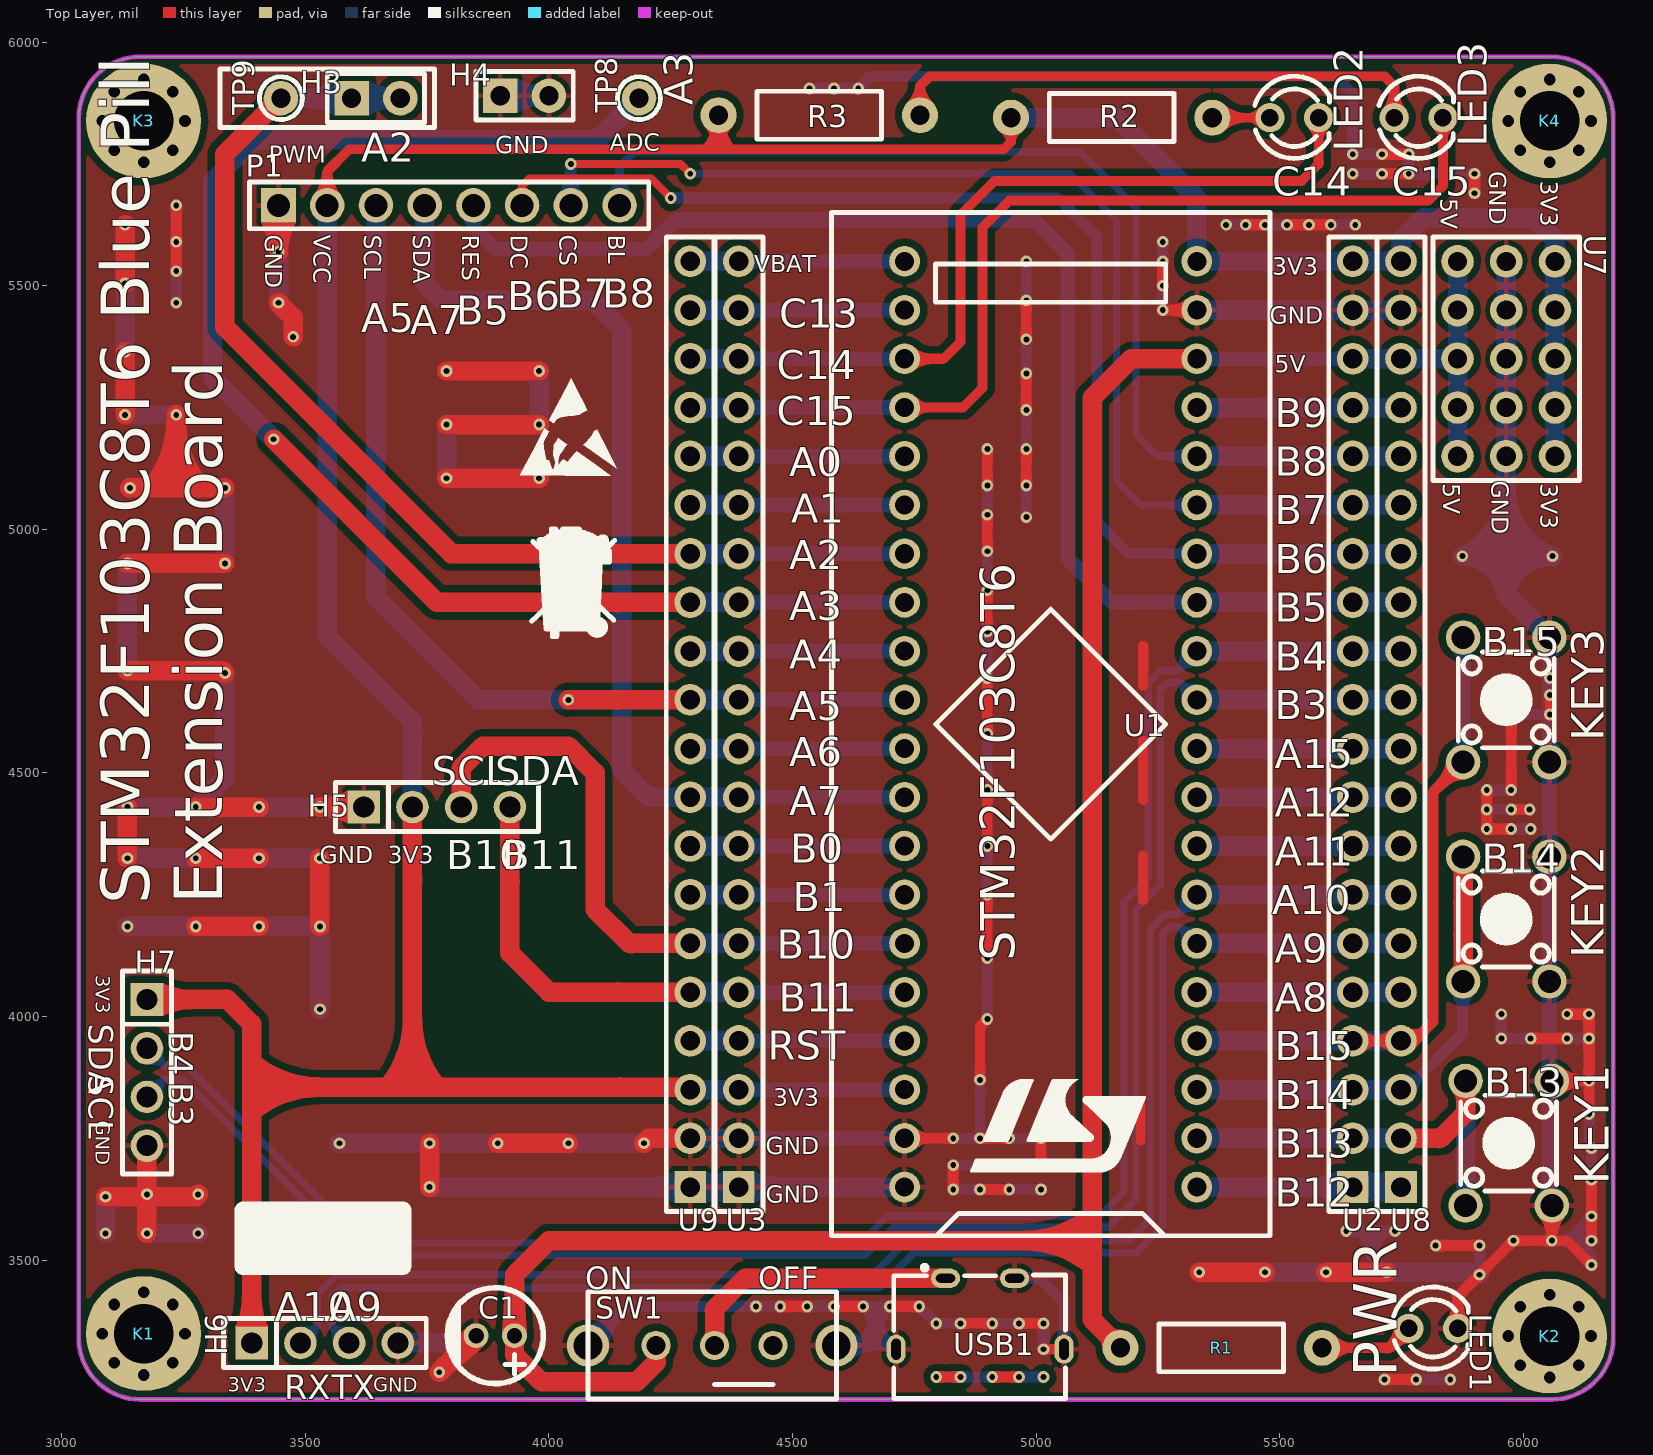
[diagram p0: Top Layer view]
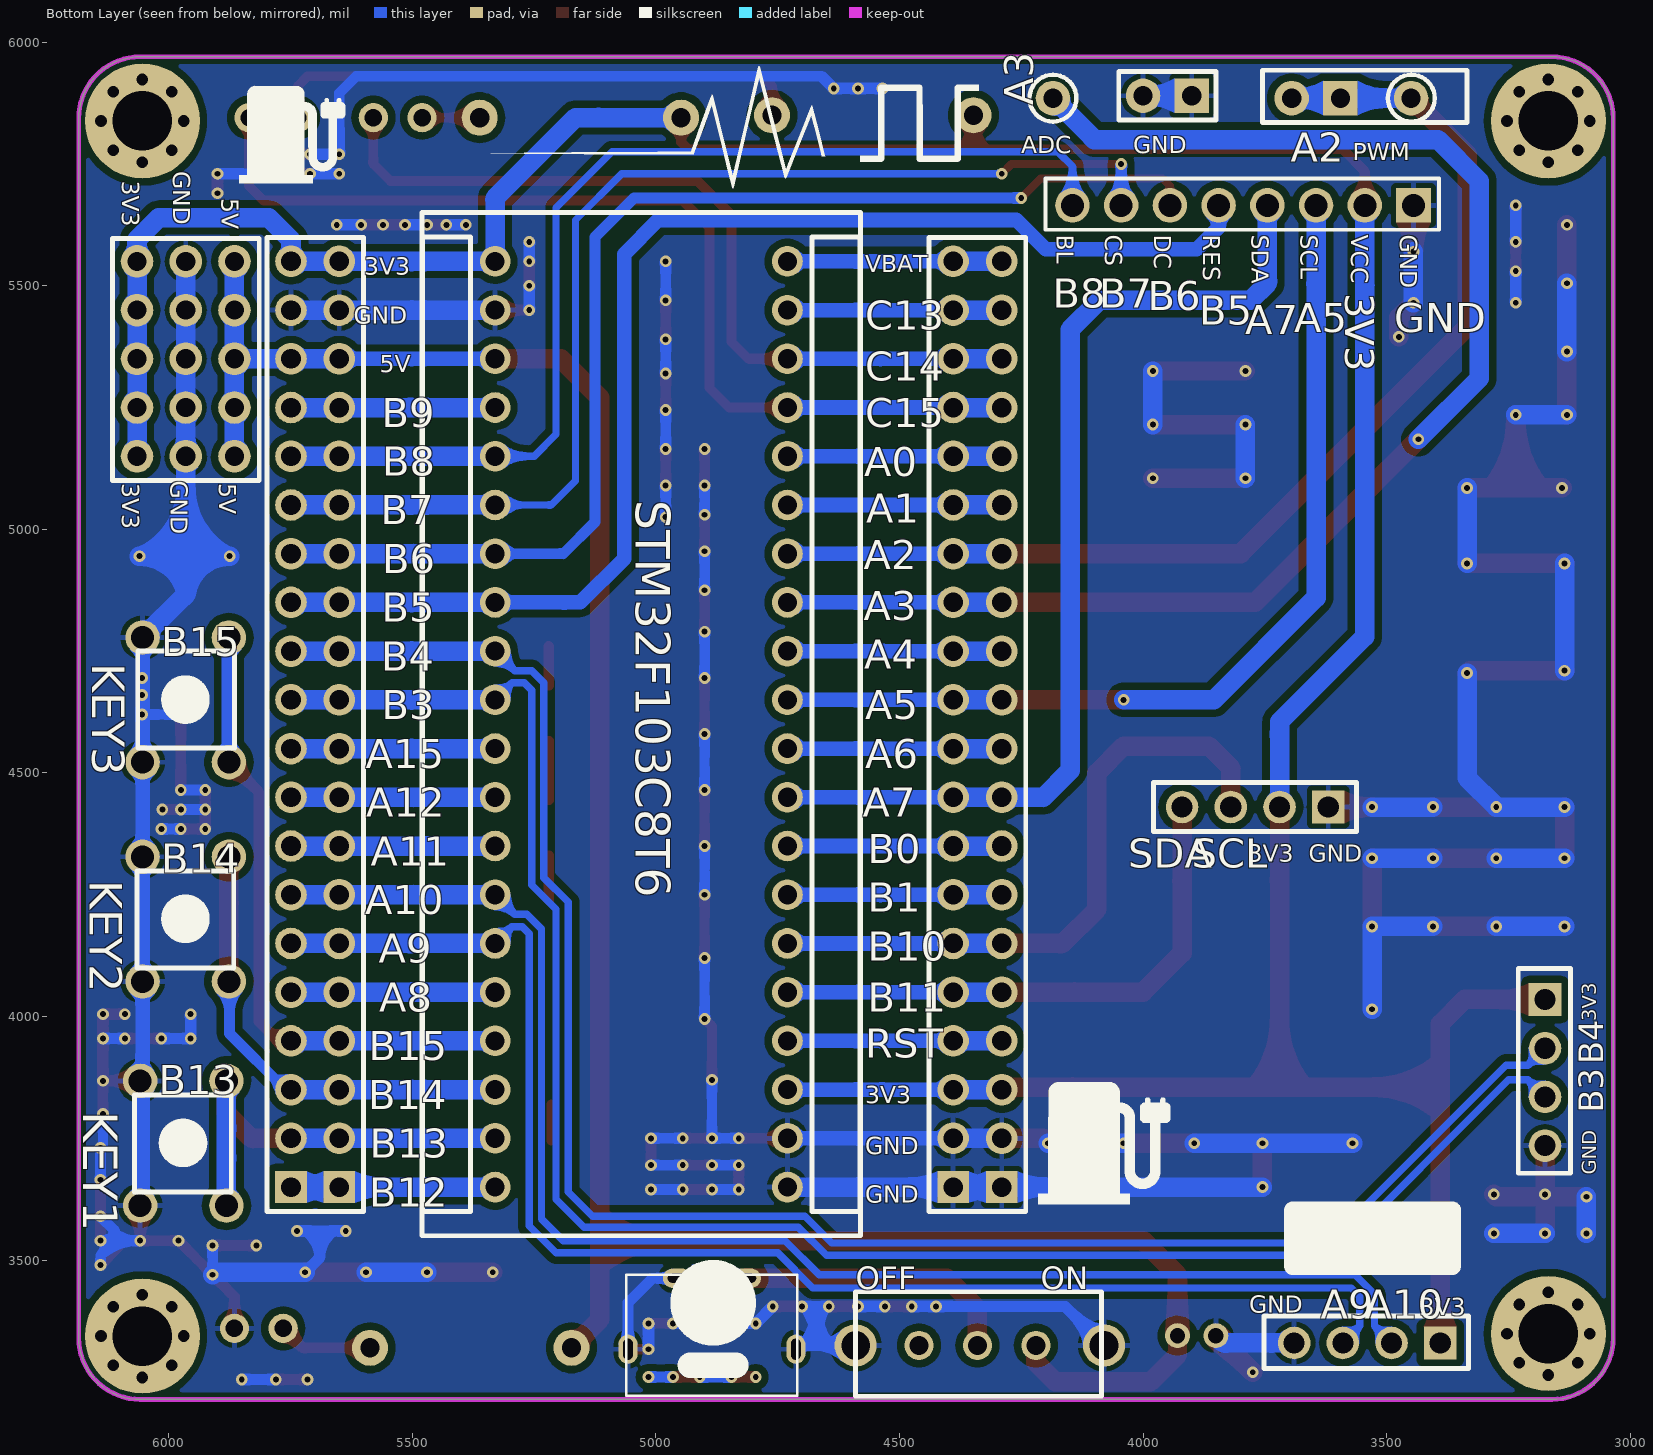
[diagram p1: Bottom Layer view, seen from below]
# Altium PCB MISC75409.pcbdoc
Units mil, origin at the board's own origin, x right, y up, seen from the top; angles counter-clockwise.
Board outline 3149.61 x 2755.91 mil, 2 copper layers (Top Layer, Bottom Layer), stack 62.206 mil thick; 30 components, 42 nets, 232 pads, 171 vias.

## Layer stack, top to bottom
Top Solder Mask Layer: solder mask 0.394, Dk 3.3
Top Layer: signal copper 1.379
Dielectric1: surface 59.449, FR4, Dk 4.5
Bottom Layer: signal copper 1.378
Bottom Solder Mask Layer: solder mask 0.394, Dk 3.3

## Board outline
3160.98,5970 ccw(c3160.98,5844.02) 3035,5844.02 3035,3340.08 ccw(c3160.98,3340.08) 3160.98,3214.09 6058.62,3214.09 ccw(c6058.62,3340.08) 6184.61,3340.08 6184.61,5844.02 ccw(c6058.62,5844.02) 6058.62,5970

## Design rules (kind name [scope] priority, off if disabled: settings)
BoardOutlineClearance copperThickness2oz_1 [All] p2 off: genericclearance=7.99 ignorepadtopadclearanceinfootprint=FALSE except(0: Arc-SplitContinuation Track-SplitContinuation SMDPad-SplitContinuation THPad-SplitContinuation Via-SplitContinuation Fill-SplitContinuation Region-SplitContinuation Poly-SplitContinuation Text-SplitContinuation Hole-SplitContinuation; 5.98: Arc-CutoutEdge Track-CutoutEdge SMDPad-CutoutEdge THPad-CutoutEdge Via-CutoutEdge Text-CutoutEdge; 6.89: Hole-OutlineEdge Hole-CutoutEdge; 11.81: Arc-OutlineEdge Track-OutlineEdge SMDPad-OutlineEdge THPad-OutlineEdge Via-OutlineEdge Fill-OutlineEdge Region-OutlineEdge Text-OutlineEdge Fill-CutoutEdge Region-CutoutEdge; 15: Poly-OutlineEdge Poly-CutoutEdge)
BoardOutlineClearance Plane_innerPlane_1 [All] p4 off: genericclearance=4.02 ignorepadtopadclearanceinfootprint=FALSE except(0: Arc-SplitContinuation Track-SplitContinuation SMDPad-SplitContinuation THPad-SplitContinuation Via-SplitContinuation Fill-SplitContinuation Region-SplitContinuation Poly-SplitContinuation Text-SplitContinuation Hole-SplitContinuation; 5.98: Arc-CutoutEdge Track-CutoutEdge SMDPad-CutoutEdge THPad-CutoutEdge Via-CutoutEdge Text-CutoutEdge; 6.89: Hole-OutlineEdge Hole-CutoutEdge; 10: Poly-OutlineEdge Poly-CutoutEdge; 11.81: Arc-OutlineEdge Track-OutlineEdge SMDPad-OutlineEdge THPad-OutlineEdge Via-OutlineEdge Fill-OutlineEdge Region-OutlineEdge Text-OutlineEdge Fill-CutoutEdge Region-CutoutEdge)
BoardOutlineClearance Copper_copperRegion_1 [All] p6 off: genericclearance=4.02 ignorepadtopadclearanceinfootprint=FALSE except(0: Arc-SplitContinuation Track-SplitContinuation SMDPad-SplitContinuation THPad-SplitContinuation Via-SplitContinuation Fill-SplitContinuation Region-SplitContinuation Poly-SplitContinuation Text-SplitContinuation Hole-SplitContinuation; 5.98: Arc-CutoutEdge Track-CutoutEdge SMDPad-CutoutEdge THPad-CutoutEdge Via-CutoutEdge Text-CutoutEdge; 6.89: Hole-OutlineEdge Hole-CutoutEdge; 11.81: Arc-OutlineEdge Track-OutlineEdge SMDPad-OutlineEdge THPad-OutlineEdge Via-OutlineEdge Fill-OutlineEdge Region-OutlineEdge Text-OutlineEdge Fill-CutoutEdge Region-CutoutEdge; 15: Poly-OutlineEdge Poly-CutoutEdge)
BoardOutlineClearance copperThickness1oz_1 [All] p8: genericclearance=4.02 ignorepadtopadclearanceinfootprint=FALSE except(0: Arc-SplitContinuation Track-SplitContinuation SMDPad-SplitContinuation THPad-SplitContinuation Via-SplitContinuation Fill-SplitContinuation Region-SplitContinuation Poly-SplitContinuation Text-SplitContinuation Hole-SplitContinuation; 5.98: Arc-CutoutEdge Track-CutoutEdge SMDPad-CutoutEdge THPad-CutoutEdge Via-CutoutEdge Text-CutoutEdge; 6.89: Hole-OutlineEdge Hole-CutoutEdge; 11.81: Arc-OutlineEdge Track-OutlineEdge SMDPad-OutlineEdge THPad-OutlineEdge Via-OutlineEdge Fill-OutlineEdge Region-OutlineEdge Text-OutlineEdge Fill-CutoutEdge Region-CutoutEdge; 15: Poly-OutlineEdge Poly-CutoutEdge)
Clearance copperThickness2oz [All] p1 off: gap=7.99 ignorepadtopadclearanceinfootprint=FALSE except(5.98: SMDPad-Track SMDPad-SMDPad THPad-Track SMDPad-THPad THPad-THPad Track-Via SMDPad-Via THPad-Via Via-Via Fill-SMDPad Region-SMDPad Fill-THPad Region-THPad Fill-Via Region-Via Fill-Fill Fill-Region Region-Region Arc-Track Arc-SMDPad Arc-THPad Arc-Via Fill-Arc Region-Arc Arc-Arc Text-Track SMDPad-Text Text-THPad Text-Via Fill-Text Region-Text Arc-Text Text-Text; 6.89: Hole-Track Hole-SMDPad Hole-THPad Hole-Via Fill-Hole Region-Hole Hole-Arc Hole-Text; 11.81: Fill-Track Region-Track; 15: Poly-Track Poly-SMDPad Poly-THPad Poly-Via Poly-Fill Poly-Region Poly-Poly Poly-Arc Poly-Text Poly-Hole)
Clearance Plane_innerPlane [All] p3 off: gap=4.02 ignorepadtopadclearanceinfootprint=FALSE except(5.98: SMDPad-Track SMDPad-SMDPad THPad-Track SMDPad-THPad THPad-THPad Track-Via SMDPad-Via THPad-Via Via-Via Fill-SMDPad Region-SMDPad Fill-THPad Region-THPad Fill-Via Region-Via Fill-Fill Fill-Region Region-Region Arc-Track Arc-SMDPad Arc-THPad Arc-Via Fill-Arc Region-Arc Arc-Arc Text-Track SMDPad-Text Text-THPad Text-Via Fill-Text Region-Text Arc-Text Text-Text; 6.89: Hole-Track Hole-SMDPad Hole-THPad Hole-Via Fill-Hole Region-Hole Hole-Arc Hole-Text; 10: Poly-Track Poly-SMDPad Poly-THPad Poly-Via Poly-Fill Poly-Region Poly-Poly Poly-Arc Poly-Text Poly-Hole; 11.81: Fill-Track Region-Track)
Clearance Copper_copperRegion [All] p5 off: gap=4.02 ignorepadtopadclearanceinfootprint=FALSE except(5.98: SMDPad-Track SMDPad-SMDPad THPad-Track SMDPad-THPad THPad-THPad Track-Via SMDPad-Via THPad-Via Via-Via Fill-SMDPad Region-SMDPad Fill-THPad Region-THPad Fill-Via Region-Via Fill-Fill Fill-Region Region-Region Arc-Track Arc-SMDPad Arc-THPad Arc-Via Fill-Arc Region-Arc Arc-Arc Text-Track SMDPad-Text Text-THPad Text-Via Fill-Text Region-Text Arc-Text Text-Text; 6.89: Hole-Track Hole-SMDPad Hole-THPad Hole-Via Fill-Hole Region-Hole Hole-Arc Hole-Text; 11.81: Fill-Track Region-Track; 15: Poly-Track Poly-SMDPad Poly-THPad Poly-Via Poly-Fill Poly-Region Poly-Poly Poly-Arc Poly-Text Poly-Hole)
Clearance copperThickness1oz [All] p7: gap=4.02 ignorepadtopadclearanceinfootprint=FALSE except(5.98: SMDPad-Track SMDPad-SMDPad THPad-Track SMDPad-THPad THPad-THPad Track-Via SMDPad-Via THPad-Via Via-Via Fill-SMDPad Region-SMDPad Fill-THPad Region-THPad Fill-Via Region-Via Fill-Fill Fill-Region Region-Region Arc-Track Arc-SMDPad Arc-THPad Arc-Via Fill-Arc Region-Arc Arc-Arc Text-Track SMDPad-Text Text-THPad Text-Via Fill-Text Region-Text Arc-Text Text-Text; 6.89: Hole-Track Hole-SMDPad Hole-THPad Hole-Via Fill-Hole Region-Hole Hole-Arc Hole-Text; 11.81: Fill-Track Region-Track; 15: Poly-Track Poly-SMDPad Poly-THPad Poly-Via Poly-Fill Poly-Region Poly-Poly Poly-Arc Poly-Text Poly-Hole)
DiffPairsRouting differentialPair [All] p1: maxlimit=6 minlimit=6 mostfreqgap=6 toplayer_minwidth=5 toplayer_prefwidth=10 toplayer_maxwidth=100 toplayer_mingap=6 toplayer_prefgap=6 toplayer_maxgap=6 bottomlayer_minwidth=5 bottomlayer_prefwidth=10 bottomlayer_maxwidth=100 bottomlayer_mingap=6 bottomlayer_prefgap=6 bottomlayer_maxgap=6 maxuncoupledlength=10
HoleToHoleClearance otherClearance [All] p1: gap=11.81 allowstackedmicrovias=TRUE
Length netLength [All] p1: minlimit=0 maxlimit=0
PasteMaskExpansion pasteMaskExpansion [All] p1: expansion=0
PlaneConnect innerPlane [All] p1: planeconnectstyle=Relief reliefexpansion=20 reliefentries=4 reliefconductorwidth=10 reliefairgap=10
PolygonConnect copperRegion [All] p1: connectstyle=Relief reliefconductorwidth=10 reliefentries=4 polygonreliefangle="90 Angle" airgapwidth=10 via.connectstyle=Relief via.reliefconductorwidth=10 via.reliefentries=4 via.polygonreliefangle="90 Angle" via.airgapwidth=10
RoutingVias viaSize [All] p1: holewidth=12.01 width=24.02 viastyle="Through Hole" minholewidth=11.81 minwidth=19.68 maxholewidth=248.03 maxwidth=393.7
SolderMaskExpansion solderMaskExpansion [IsVia] p1: expansion=-1000 istentingtop=TRUE
SolderMaskExpansion solderMaskExpansion [All] p2: expansion=2.01 istentingtop=FALSE
Width copperThickness2oz_2 [All] p1 off: maxlimit=100 minlimit=8 preferedwidth=10
Width copperThickness1oz_2 [All] p2: maxlimit=100 minlimit=5 preferedwidth=10

## Components (designator, comment, footprint, x,y, rotation, side; value= is the part's Value field where it differs from the comment)
C1 "10uF" CAP-TH_BD5.0-P2.00-D0.8-FD 3890,3345 r180 top
H3 "" HDR-TH_2P-P2.54-V-M-1 3645,5885 r0 top
H4 "" HDR-TH_2P-P2.54-V-M-1 3950,5890 r0 top
H5 "2.54-1*4P female" HDR-TH_4P-P2.54-V-F 3770,4430 r0 top
H6 "2.54-1*4P female" HDR-TH_4P-P2.54-V-F 3540,3330 r0 top
H7 "2.54-1*4P female" HDR-TH_4P-P2.54-V-F 3175,3885 r270 top
K1 "Flange pad" 法兰焊盘-8孔-M3 3168.11,3349.13 r0 top
K2 "Flange pad" 法兰焊盘-8孔-M3 6054.02,3344.13 r0 top
K3 "Flange pad" 法兰焊盘-8孔-M3 3168.11,5838.23 r0 top
K4 "Flange pad" 法兰焊盘-8孔-M3 6054.02,5838.23 r0 top
KEY1 "TC-6610-9-260G" SW-TH_4P-L5.0-W5.0-P4.50-LS6.5 5970,3740 r90 top
KEY2 "TC-6610-9-260G" SW-TH_4P-L5.0-W5.0-P4.50-LS6.5 5965,4200 r90 top
KEY3 "TC-6610-9-260G" SW-TH_4P-L5.0-W5.0-P4.50-LS6.5 5965,4650 r90 top
LED1 "" LED_TH-3mm 5815,3360 r0 top
LED2 "" LED_TH-3mm 5530,5845 r0 top
LED3 "" LED_TH-3mm 5785,5845 r0 top
P1 "2.54-1*8P female RoHS" HDR-TH_8P-P2.54-V-F-1 3795,5665 r0 top
R1 "1kΩ" RES-TH_BD2.5-L6.5-P10.50-D0.6 5380,3320 r180 top
R2 "1kΩ" RES-TH_BD2.5-L6.5-P10.50-D0.6 5155,5845 r180 top
R3 "1kΩ" RES-TH_BD2.5-L6.5-P10.50-D0.6 4555,5850 r180 top
SW1 "SK-12E12-G5" SW-TH_SK-12E12-G5 4335,3325 r270 top
TP8 "TP-yellow test point" TESTPOINT-TH_BD3.2 4185,5885 r0 top
TP9 "TP-yellow test point" TESTPOINT-TH_BD3.2 3450,5885 r0 top
U1 "LCKFB-DKX-STM32F103C8T6" CONN-TH_L53.3-W22.9_STM32F103C8T6-CARD 5030,4600 r90 top
U2 "KH-2.54FH-1X20P-H8.5" HDR-TH_20P-P2.54-V-F-2 5650,4600 r90 top
U3 "KH-2.54FH-1X20P-H8.5" HDR-TH_20P-P2.54-V-F-2 4390,4600 r90 top
U7 "HX PZ2.54-3x5P ZZ" HDR-TH_15P-P2.54-V-M-R3-C5-S7.5 5965,5350 r270 top
U8 "KH-2.54FH-1X20P-H8.5" HDR-TH_20P-P2.54-V-F-2 5749,4600 r90 top
U9 "KH-2.54FH-1X20P-H8.5" HDR-TH_20P-P2.54-V-F-2 4290,4600 r90 top
USB1 "KH-TYPE-C-2P" USB-SMD_KH-TYPE-C-2P 4885,3390 r0 top

## Footprints (in the part's own frame and the unit in brackets; to place one, negate y for a bottom-side part, rotate by r counter-clockwise, add the part's x,y. Pads: shape width x height; smd on the part's side, far side on the other; paste and mask are expansions set on the pad)
CAP-TH_BD5.0-P2.00-D0.8-FD [mm]
  round 1.3 hole 0.8: 1(-1,0) 2(1,0)
  silkscreen extent -2.5,-2.5 2.5,2.5
CONN-TH_L53.3-W22.9_STM32F103C8T6-CARD [mm]
  round 1.6 hole 1: 1(-24.13,-7.62) 2(-21.59,-7.62) 3(-19.05,-7.62) 4(-16.51,-7.62) 5(-13.97,-7.62) 6(-11.43,-7.62) 7(-8.89,-7.62) 8(-6.35,-7.62) 9(-3.81,-7.62) 10(-1.27,-7.62) 11(1.27,-7.62) 12(3.81,-7.62) 13(6.35,-7.62) 14(8.89,-7.62) 15(11.43,-7.62) 16(13.97,-7.62) 17(16.51,-7.62) 18(19.05,-7.62) 19(21.59,-7.62) 20(24.13,-7.62) 21(24.13,7.62) 22(21.59,7.62) 23(19.05,7.62) 24(16.51,7.62) 25(13.97,7.62) 26(11.43,7.62) 27(8.89,7.62) 28(6.35,7.62) 29(3.81,7.62) 30(1.27,7.62) 31(-1.27,7.62) 32(-3.81,7.62) 33(-6.35,7.62) 34(-8.89,7.62) 35(-11.43,7.62) 36(-13.97,7.62) 37(-16.51,7.62) 38(-19.05,7.62) 39(-21.59,7.62) 40(-24.13,7.62)
  silkscreen extent -26.67,-11.43 26.67,11.43
HDR-TH_2P-P2.54-V-M-1 [mm]
  rect 1.8x1.8 hole 1 paste+0 mask+0.051: 1(-1.27,0)
  round 1.8 hole 1 paste+0 mask+0.051: 2(1.27,0)
  silkscreen extent -2.54,-1.27 2.54,1.27
HDR-TH_4P-P2.54-V-F [mm]
  rect 1.7x1.7 hole 1.1: 1(-3.81,0)
  round 1.7 hole 1.1: 2(-1.27,0) 3(1.27,0) 4(3.81,0)
  silkscreen extent -5.29,-1.27 5.29,1.27
HDR-TH_8P-P2.54-V-F-1 [mm]
  rect 1.8x1.8 hole 1.2: 1(-8.89,0)
  round 1.8 hole 1.2: 2(-6.35,0) 3(-3.81,0) 4(-1.27,0) 5(1.27,0) 6(3.81,0) 7(6.35,0) 8(8.89,0)
  silkscreen extent -10.41,-1.22 10.41,1.22
HDR-TH_15P-P2.54-V-M-R3-C5-S7.5 [mm]
  round 1.7 hole 1: 1(-5.08,-2.54) 2(-5.08,0) 3(-5.08,2.54) 4(-2.54,-2.54) 5(-2.54,0) 6(-2.54,2.54) 7(0,-2.54) 8(0,0) 9(0,2.54) 10(2.54,-2.54) 11(2.54,0) 12(2.54,2.54) 13(5.08,-2.54) 14(5.08,0) 15(5.08,2.54)
  silkscreen extent -6.35,-3.81 6.35,3.81
HDR-TH_20P-P2.54-V-F-2 [mm]
  rect 1.65x1.65 hole 1.02: 1(-24.13,0)
  round 1.65 hole 1.02: 2(-21.59,0) 3(-19.05,0) 4(-16.51,0) 5(-13.97,0) 6(-11.43,0) 7(-8.89,0) 8(-6.35,0) 9(-3.81,0) 10(-1.27,0) 11(1.27,0) 12(3.81,0) 13(6.35,0) 14(8.89,0) 15(11.43,0) 16(13.97,0) 17(16.51,0) 18(19.05,0) 19(21.59,0) 20(24.13,0)
  silkscreen extent -25.4,-1.25 25.4,1.25
LED_TH-3mm [mil]
  round 60 hole 36 paste+0 mask+2: 1(-50,0) 2(50,0)
  silkscreen extent -81,-84 72,85
RES-TH_BD2.5-L6.5-P10.50-D0.6 [mil]
  round 74 hole 39.37: 1(-206.69,0) 2(206.69,0)
  silkscreen extent -128,-49 128,49
SW-TH_4P-L5.0-W5.0-P4.50-LS6.5 [mm]
  round 1.8 hole 1.2: 1(-3.25,2.25) 2(3.25,2.25) 3(-3.25,-2.25) 4(3.25,-2.25)
  silkscreen extent -2.5,-2.5 2.5,2.5
SW-TH_SK-12E12-G5 [mil]
  round 60 hole 39.37: 1(0,125) 2(0,5) 3(0,-115)
  round 86.61 hole 59.06: 4(0,-255) 5(0,255)
  silkscreen extent -110,-255 110,255
TESTPOINT-TH_BD3.2 [mm]
  round 1.8 hole 1 paste+0 mask+0.05: 1(0,0)
  silkscreen extent -1.12,-1.12 1.12,1.12
USB-SMD_KH-TYPE-C-2P [mm]
  oval 1.524x1 hole 0.45 slot 1 at 0 deg paste+0 mask+0.05: 1(-1.8,1.85) 2(1.8,1.85)
  oval 1x1.524 hole 0.5 slot 1.1 at 90 deg paste+0 mask+0.05: 3(4.375,-1.85) 4(-4.375,-1.85)
  silkscreen extent -4.5,-4.41 4.46,2.53
法兰焊盘-8孔-M3 [mm]
  round 1 hole 0.61 paste+0 mask+0: 1(-2.159,0) 1(-1.524,-1.524) 1(-1.524,1.524) 1(0,-2.159) 1(0,2.159) 1(1.524,-1.524) 1(1.524,1.524) 1(2.159,0)
  round 6 hole 3.1 paste+0 mask+0.102: 1(0,0)

## Via types
v1: diameter 24, hole 12, Top Layer to Bottom Layer, 171 vias

## Nets (pads, with @x,y where several pads share a name; then routed paths per layer and width w, separated by ;. In a path a pad name is that pad's centre, name@x,y a point inside that pad or via, vN(x,y) a via of type N, cw(c..) or ccw(c..) an arc to the next point about the centre after c; other vN are vias at no path point)
3V3: H5.2 H6.1 H7.1 P1.2 R2.2 R3.2 U1.20 U1.38 U2.20 U3.3 U7.3 U7.6 U7.9 U7.12 U7.15 U8.20 U9.3 | length 7575.2
  Top Layer w20: P1.2 3545,5735 3590,5780 4348.31,5780 ; R3.2 4348.31,5780 ; R2.2 4948.31,5795 4933.31,5780 4348.31,5780
  Top Layer w40: H7.1 3340,4035 3390,3985 3390,3855 ; H6.1 3390,3855 ; H5.2 3720,3855 ; U9.3 4285,3855 3720,3855 ; 3390,3855 3720,3855
  Bottom Layer w30: U3.3 U1.38
  Bottom Layer w40: P1.2 3545,4780 3720,4605 H5.2 ; U9.3 U3.3 ; R2.2 5165,5845 5330,5680 U1.20 U2.20 U8.20 5749,5594 5795,5640 6020,5640 6065,5595 U7.3 U7.6 U7.9 U7.12 U7.15
$1N1650: LED2.1 R2.1 | length 118.3
  Top Layer w20: R2.1 LED2.1
$1N1651: LED3.1 R3.1 | length 1114.9
  Top Layer w20: R3.1 4761.69,5910 4781.69,5930 5715,5930 5735,5910 LED3.1
$1N2733: LED1.1 R1.1 | length 194.9
  Top Layer w22: R1.1 5725,3320 LED1.1
$1N2736: SW1.2 USB1.1 | length 575.2
  Top Layer w40: SW1.2 4340,3400 4402.84,3462.84 USB1.1
+5V: C1.1 R1.2 SW1.3 U1.18 U2.18 U7.1 U7.4 U7.7 U7.10 U7.13 U8.18 | length 4901.2
  Top Layer w40: SW1.3 4220,3290 4180,3250 3985,3250 3929.37,3305.63 C1.1 3929.37,3469.37 4000,3540 5115,3540 ; R1.2 5115,3378.31 5115,3540 ; U1.18 5195,5350 5115,5270 5115,3540
  Bottom Layer w30: U1.18 U2.18
  Bottom Layer w40: U2.18 5750,5350 U7.7 ; U7.13 U7.10 U7.7 ; U7.1 U7.4 U7.7
A0: U1.25 U3.16 U9.16 | length 440
  Bottom Layer w30: U3.16 U1.25
  Bottom Layer w40: U9.16 U3.16
A1: U1.26 U3.15 U9.15 | length 440
  Bottom Layer w30: U3.15 U1.26
  Bottom Layer w40: U9.15 U3.15
A2: H3.1 H3.2 TP9.1 U1.27 U3.14 U9.14 | length 2350.2
  Top Layer w40: TP9.1 3335,5770 3335,5415 3800,4950 U9.14
  Bottom Layer w30: U3.14 U1.27
  Bottom Layer w40: TP9.1 H3.1 H3.2 ; U9.14 U3.14
A3: TP8.1 U1.28 U3.13 U9.13 | length 2961
  Top Layer w40: v1(3435,5185) 3770,4850 U9.13
  Bottom Layer w30: U3.13 U1.28
  Bottom Layer w40: v1(3435,5185) 3310,5310 3310,5715 3395,5800 4100,5800 TP8.1 ; U9.13 U3.13
A4: U1.29 U3.12 U9.12 | length 440
  Bottom Layer w30: U3.12 U1.29
  Bottom Layer w40: U9.12 U3.12
A5: P1.3 U1.30 U3.11 U9.11 | length 1977
  Top Layer w40: v1(4040,4650) U9.11
  Bottom Layer w30: U3.11 U1.30
  Bottom Layer w40: P1.3 3645,4860 3855,4650 v1(4040,4650) ; U9.11 U3.11
A6: U1.31 U3.10 U9.10 | length 440
  Bottom Layer w30: U3.10 U1.31
  Bottom Layer w40: U9.10 U3.10
A7: P1.4 U1.32 U3.9 U9.9 | length 2112.1
  Bottom Layer w30: U3.9 U1.32
  Bottom Layer w40: P1.4 3745,5505 3780,5470 4090,5470 4150,5410 4150,4505 4205,4450 U9.9 U3.9
A8: U1.5 U2.5 U8.5 | length 419
  Bottom Layer w40: U1.5 U2.5 U8.5
A9: H6.3 U1.6 U2.6 U8.6 | length 2983.8
  Bottom Layer w15: H6.3 3555,3365 3555,3425 3573,3443 4678,3443 4750,3515 5205,3515 5260,3570 5260,4170 5274.39,4184.39 5295.61,4184.39 U1.6
  Bottom Layer w40: U1.6 U2.6 U8.6
A10: H6.2 U1.7 U2.7 U8.7 | length 3026.7
  Bottom Layer w15: H6.2 3525,3365 3525,3430 3565,3470 4665,3470 4735,3540 5190,3540 5235,3585 5235,4180 5265,4210 5290,4210 U1.7
  Bottom Layer w40: U1.7 U2.7 U8.7
A11: U1.8 U2.8 U8.8 | length 415
  Bottom Layer w40: U1.8 5636.28,4350 U2.8@5643.14,4343.14 ; U2.8 U8.8
A12: U1.9 U2.9 U8.9 | length 417.9
  Bottom Layer w40: U1.9 5646.28,4450 U2.9@5648.14,4451.86 ; U2.9 U8.9
A15: U1.10 U2.10 U8.10 | length 419
  Bottom Layer w40: U1.10 U2.10 U8.10
AGND:  | length 220
  Top Layer w22: v1(4795,3260) v1(4845,3260) ; v1(4910,3260) v1(4965,3260)
  Bottom Layer w22: v1(4845,3260) v1(4910,3260) ; v1(4965,3260) v1(5015,3260)
B0: U1.33 U3.8 U9.8 | length 440
  Bottom Layer w30: U3.8 U1.33
  Bottom Layer w40: U9.8 U3.8
B1: U1.34 U3.7 U9.7 | length 440
  Bottom Layer w30: U3.7 U1.34
  Bottom Layer w40: U9.7 U3.7
B3: H7.3 U1.11 U2.11 U8.11 | length 3820.6
  Bottom Layer w15: H7.3 3210,3870 3250,3870 3610,3510 4650,3510 4707.52,3567.52 5147.52,3567.52 5205,3625 5205,4220 5255,4270 5255,4670 5270,4685 5295,4685 U1.11
  Bottom Layer w40: U1.11 5646.28,4650 U2.11@5648.14,4651.86 ; U2.11 U8.11
B4: H7.2 U1.12 U2.12 U8.12 | length 3825.8
  Bottom Layer w15: H7.2 3210,3900 3255,3900 3620,3535 4638.89,3535 4693.89,3590 5130,3590 5180,3640 5180,4235 5230,4285 5230,4685 5255,4710 5290,4710 U1.12
  Bottom Layer w40: U1.12 U2.12 U8.12
B5: P1.5 U1.13 U2.13 U8.13 | length 2683.8
  Bottom Layer w30: P1.5 3845,5620 3890,5575 4200,5575 4260,5635 4995,5635 5065,5565 5065,4940 5155,4850 U1.13
  Bottom Layer w40: U1.13 U2.13 U8.13
B6: P1.6 U1.14 U2.14 U8.14 | length 2511.8
  Top Layer w16: P1.6 3945,5705 3960,5720 4210,5720 v1(4250,5680)
  Bottom Layer w22: v1(4250,5680) 5045,5680 5125,5600 5125,5015 5190,4950 U1.14
  Bottom Layer w40: U1.14 U2.14 U8.14
B7: P1.7 U1.15 U2.15 U8.15 | length 2392.3
  Top Layer w16: v1(4045,5750) 4270,5750 v1(4290,5730)
  Bottom Layer w15: v1(4290,5730) 5070,5730 5165,5635 5165,5100 5215,5050 U1.15
  Bottom Layer w22: P1.7 v1(4045,5750)
  Bottom Layer w40: U1.15 U2.15 U8.15
B8: P1.8 U1.16 U2.16 U8.16 | length 2227.7
  Bottom Layer w15: P1.8 4145,5745 4175,5775 5090,5775 5205,5660 5205,5195 5250,5150 U1.16
  Bottom Layer w40: U1.16 U2.16 U8.16
B9: U1.17 U2.17 U8.17 | length 419
  Bottom Layer w40: U1.17 U2.17 U8.17
B10: H5.3 U1.35 U3.6 U9.6 | length 1341.3
  Top Layer w40: H5.3 3820,4510 3865,4555 4040,4555 4095,4500 4095,4220 4165,4150 U9.6
  Bottom Layer w15: 4629.39,4150.61 4630,4150
  Bottom Layer w30: U3.6 4630,4150 U1.35
  Bottom Layer w40: U9.6 U3.6
B11: H5.4 U1.36 U3.5 U9.5 | length 1143.1
  Top Layer w40: H5.4 3920,4130 4000,4050 U9.5
  Bottom Layer w30: U3.5 U1.36
  Bottom Layer w40: U9.5 U3.5
B12: U1.1 U2.1 U8.1 | length 419
  Bottom Layer w40: U1.1 U2.1 U8.1
B13: KEY1.1 KEY1.2 U1.2 U2.2 U8.2 | length 895.1
  Top Layer w40: U8.2 5830,3750 5881.42,3801.42 KEY1.2
  Bottom Layer w40: U1.2 U2.2 U8.2 ; KEY1.1 KEY1.2
B14: KEY2.1 KEY2.2 U1.3 U2.3 U8.3 | length 955.5
  Top Layer w40: KEY2.1 KEY2.2
  Bottom Layer w22: U8.3@5749,3851.72 5761.72,3851.72 5875,3965 5875,4070.63 KEY2.1
  Bottom Layer w40: U1.3 U2.3 U8.3
B15: KEY3.1 KEY3.2 U1.4 U2.4 U8.4 | length 1414
  Top Layer w22: U2.4 5775,3950 5815,3990 5815,4460.63 KEY3.1
  Bottom Layer w30: KEY3.1 KEY3.2
  Bottom Layer w40: U1.4 U2.4 U8.4
C13: U1.22 U3.19 U9.19 | length 440
  Bottom Layer w30: U3.19 U1.22
  Bottom Layer w40: U9.19 U3.19
C14: LED2.2 U1.23 U3.18 U9.18 | length 1703
  Top Layer w20: U1.23 4810,5350 4845,5385 4845,5645 4915,5715 5545,5715 5580,5750 LED2.2
  Bottom Layer w30: U3.18 U1.23
  Bottom Layer w40: U9.18 U3.18
C15: LED3.2 U1.24 U3.17 U9.17 | length 2066.8
  Top Layer w20: U1.24 4850,5250 4890,5290 4890,5620 4945,5675 5805,5675 5835,5705 LED3.2
  Bottom Layer w30: U3.17 U1.24
  Bottom Layer w40: U9.17 U3.17
GND: C1.2 H4.1 H4.2 H5.1 H6.4 H7.4 KEY1.3 KEY1.4 KEY2.3 KEY2.4 KEY3.3 KEY3.4 LED1.2 P1.1 SW1.4 SW1.5 U1.19 U1.39 U1.40 U2.19 U3.1 U3.2 U7.2 U7.5 U7.8 U7.11 U7.14 U8.19 U9.1 U9.2 USB1.2 USB1.3 USB1.4 | length 20619.9
  Top Layer w20: v1(3235,5530) v1(3235,5590) ; U1.39 v1(4830,3750) ; v1(4830,3645) v1(4830,3695) ; v1(4845,3370) v1(4910,3370) ; v1(4885,3645) v1(4945,3645) ; v1(4885,3695) v1(4945,3695) ; v1(4885,3750) v1(4945,3750) ; v1(4885,3870) 4885,3980 v1(4900,3995) ; v1(4900,4120) v1(4900,4250) ; v1(4900,4350) v1(4900,4465) ; v1(4900,4580) v1(4900,4695) ; v1(4900,4790) v1(4900,4875) ; v1(4900,4955) v1(4900,5030) ; v1(4900,5090) v1(4900,5165) ; v1(4965,3370) v1(5015,3370) ; v1(4980,5090) v1(4980,5165) ; v1(4980,5245) v1(4980,5320) ; v1(4980,5390) v1(4980,5470) ; v1(5010,3695) v1(5010,3750) ; v1(5015,3317.16) 5042.24,3317.16 USB1.3@5067.24,3317.16 ; 5215,3745 5215,3820 ; v1(5260,5450) U1.19 ; v1(5910,3470) v1(5980,3540) v1(6058.58,3540) ; v1(5925,4425) v1(5925,4465) ; v1(5975,4425) v1(6012.95,4425) ; v1(6055,4620) v1(6055,4660) ; KEY1.3 v1(6058.58,3540) ; KEY1.4 6133.21,3867.95 v1(6135,3867.95) v1(6135,3800) ; v1(6140,3490) 6090,3540 v1(6058.58,3540) ; v1(6140,3540) v1(6140,3590) v1(6140,3665)
  Top Layer w22: v1(3235,5590) v1(3235,5665) ; v1(4475,3405) v1(4530,3405) ; v1(4585,3405) v1(4645,3405) ; v1(4700,3405) v1(4760,3405) ; 5220,4240 5220,4330 ; 5220,4445 5220,4565 ; 5220,4680 5220,4760 ; v1(5260,5500) v1(5260,5550) ; v1(5430,5625) v1(5470,5625) ; v1(5515,5625) v1(5560,5625) v1(5605,5625) ; v1(5710,5730) v1(5765,5730) ; v1(5710,5770) v1(5765,5770) ; v1(5715,3255) v1(5780,3255) ; v1(5820,3530) v1(5910,3530) ; LED1.2 5865,3425 v1(5910,3470) ; v1(5900,5690) v1(5900,5730) ; v1(5925,4425) v1(5925,4385) v1(5975,4385) ; v1(5975,4465) v1(5975,4620) ; v1(6015,3955) v1(6090,3955) ; v1(6090,4005) v1(6135,4005) v1(6135,3955) 6135,3869.74 v1@6133.21,3867.95
  Top Layer w40: v1(3090,3630) v1@3175,3630 ; v1(3130,5235) v1(3130,5365) ; v1(3130,5505) v1(3130,5625) ; v1(3135,4325) v1(3135,4430) ; v1(3135,4710) 3330,4710 v1(3335,4705) ; v1(3135,4930) v1(3335,4930) ; v1(3140,5085) 3234.61,5085 ; v1(3175,3555) v1@3175,3630 ; H7.4 v1(3175,3635) v1@3175,3630 ; v1(3235,5235) 3235,5085.39 3234.61,5085 ; v1(3275,4185) v1(3405,4185) ; v1(3275,4325) v1(3405,4325) ; v1(3275,4430) v1(3405,4430) ; v1(3280,3635) 3275,3630 v1@3175,3630 ; v1(3335,5085) 3234.61,5085 ; v1(3445,5465) 3475,5435 v1(3475,5395) ; v1(3445,5570) P1.1 ; v1(3530,4185) v1(3530,4325) ; v1(3530,4430) H5.1 ; v1(3755,3650) v1(3755,3740) ; v1(3775,3270) 3850,3345 C1.2 ; v1(3790,5105) v1(3980,5105) ; v1(3790,5215) v1(3980,5215) ; v1(3790,5325) v1(3980,5325) ; v1(3895,3740) v1(4040,3740) ; v1(4195,3740) 4205,3750 U9.2 ; v1(5335,3475) v1(5470,3475) ; v1(5595,3475) v1(5720,3475)
  Bottom Layer w20: v1(4795,3370) v1(4845,3370) ; v1(4830,3645) v1(4885,3645) ; v1(4830,3695) v1(4885,3695) ; v1(4830,3750) v1(4885,3750) v1(4885,3870) ; v1(4900,3995) v1(4900,4120) ; v1(4900,4250) v1(4900,4350) ; v1(4900,4465) v1(4900,4580) ; v1(4900,4695) v1(4900,4790) ; v1(4900,4875) v1(4900,4955) ; v1(4900,5030) v1(4900,5090) ; v1(4910,3370) v1(4965,3370) ; v1(4945,3645) v1(5010,3645) ; v1(4945,3695) v1(5010,3695) ; v1(4945,3750) v1(5010,3750) ; v1(4980,5025) v1(4980,5090) ; v1(4980,5165) v1(4980,5245) ; v1(4980,5320) v1(4980,5390) ; v1(4980,5470) v1(4980,5550) ; v1(5910,3470) v1(5910,3530) ; v1(5925,4425) v1(5975,4425) ; v1(5925,4465) v1(5975,4465) ; v1(5975,4620) v1@6053.58,4620 ; v1(6058.58,3540) 6110,3540 ; v1(6135,3800) 6135,3735 v1(6140,3730) v1(6140,3665) ; v1(6140,3490) 6140,3510 6110,3540 ; v1(6140,3540) 6110,3540 ; v1(6140,3590) 6110,3560 6110,3540
  Bottom Layer w22: v1(3235,5465) v1(3235,5530) ; v1(3235,5590) v1(3235,5665) ; SW1.4 4160,3405 v1(4425,3405) v1(4475,3405) ; v1(4530,3405) v1(4585,3405) ; v1(4535,5905) v1(4585,5905) v1(4635,5905) 4660,5930 5615,5930 5650,5895 v1(5650,5770) v1(5710,5770) ; SW1.5@4600,3325 4669.17,3325 ; v1(4645,3405) 4670.55,3405 ; v1(4700,3405) 4670.55,3405 ; USB1.4@4714.92,3325 4669.17,3325 ; v1(4760,3405) v1(4795,3370) ; USB1.2@4965.86,3462.84 5007.16,3462.84 5057.24,3412.76 USB1.3 ; v1(5015,3317.16) v1(5015,3370) ; v1(5260,5450) v1(5260,5500) ; v1(5260,5550) v1(5260,5590) ; v1(5390,5625) v1(5430,5625) ; v1(5470,5625) v1(5515,5625) ; v1(5605,5625) v1(5655,5625) ; v1(5636.69,3560) 5690,3560 ; v1(5650,5730) v1(5710,5730) ; v1(5720,3475) 5690,3505 5690,3560 ; v1(5736.69,3560) 5690,3560 ; v1(5765,5770) v1(5765,5730) v1(5900,5730) ; v1(5780,3255) v1(5850,3255) ; v1(5955,4005) v1(5955,3955) v1(6015,3955) ; v1(5975,4385) v1(6015,4385) ; v1(6090,3955) v1(6135,3955) ; 4669.17,3325 4670.55,3326.38 4670.55,3405
  Bottom Layer w30: U3.2 U1.39 ; KEY3.4 6053.58,4620 KEY3.3 KEY2.4 KEY2.3 6053.58,3617.05 KEY1.3
  Bottom Layer w40: v1(3090,3555) v1(3090,3630) ; v1(3130,5235) v1(3235,5235) ; v1(3130,5365) v1(3130,5505) ; v1(3135,4185) v1(3275,4185) ; v1(3135,4325) v1(3275,4325) ; v1(3135,4430) v1(3275,4430) 3335,4490 v1(3335,4705) ; v1(3135,4710) v1(3135,4930) ; v1(3175,3555) v1(3280,3555) ; v1(3335,4930) v1(3335,5085) ; v1(3405,4185) v1(3530,4185) v1(3530,4015) ; v1(3405,4325) v1(3530,4325) ; v1(3405,4430) v1(3530,4430) ; v1(3445,5465) v1(3445,5570) ; v1(3570,3740) v1(3755,3740) v1(3895,3740) ; H6.4 3835.63,3330 C1.2 ; v1(3755,3650) U9.1 U3.1 ; v1(3790,5105) v1(3790,5215) ; H4.1 H4.2 ; v1(3980,5215) v1(3980,5325) ; v1(4040,3740) v1(4195,3740) ; U9.2 U3.2 ; U3.1@4390,3659.8 4399.8,3650 U1.40 ; U1.19 U2.19 U8.19 ; v1(5470,3475) v1(5595,3475) ; v1(5720,3475) 5905,3475 v1(5910,3470) ; v1(5875,4945) 5964.04,4945 ; U7.14 5965,5196.41 ; U7.2 U7.5 U7.8 U7.11 5965,5196.41 ; KEY3.4 5963.74,4867.79 5964.04,4945 ; v1(6060,4945) 5964.04,4945 ; 5964.04,4945 5965,5196.41
  other v1: 6055,4695
RST: U1.37 U3.4 U9.4 | length 440
  Bottom Layer w30: U3.4 U1.37
  Bottom Layer w40: U9.4 U3.4
VBAT: U1.21 U3.20 U9.20 | length 440
  Bottom Layer w30: U3.20 U1.21
  Bottom Layer w40: U9.20 U3.20
pads on no net: K1.1 K2.1 K3.1 K4.1 SW1.1

## Polygon pours and split planes (outlines as drawn)
GND on Bottom Layer (solid, remove dead copper, pour order 2): 3000,6005 3000,3185 6220,3185 6220,6005
GND on Top Layer (solid, remove dead copper, pour order 0): 3000,6005 3000,3185 6220,3185 6220,6005

## Keep-outs
Board Outline Layer:
  the board outline again, w10

## Other copper
Top Layer:
  drawing of 160 lines, arcs and shapes, not listed
Bottom Layer:
  drawing of 362 lines, arcs and shapes, not listed

## Silkscreen, mask and mechanical layers (free items; w line width, h text height)
Top Silkscreen Layer:
  drawing of 32 lines, arcs and shapes, not listed
  text "A3" at 4295,5870 h60 r90
  text "ADC" at 4125,5765 h60
  text "GND" at 3890,5760 h60
  text "A2" at 3615,5755 h60
  text "PWM" at 3425,5740 h60
  text "GND" at 5918.08,5735 h60 r270
  text "3V3" at 6023.08,5715 h60 r270
  text "C14" at 5485,5685 h60
  text "C15" at 5730,5685 h60
  text "5V" at 5818.08,5680 h60 r270
  text "GND" at 3405,5605 h60 r270
  text "VCC" at 3505,5605 h60 r270
  text "SCL" at 3608.74,5605 h60 r270
  text "SDA" at 3709.03,5605 h60 r270
  text "RES" at 3809.33,5605 h60 r270
  text "DC" at 3909.74,5605 h60 r270
  text "CS" at 4009.96,5605 h60 r270
  text "BL" at 4109.06,5605 h60 r270
  text "VBAT" at 4421,5515.36 h60
  text "3V3" at 5485,5510 h60
  text "B7" at 4015,5455 h60
  text "B8" at 4110,5455 h60
  text "B6" at 3915,5450 h60
  text "B5" at 3810,5420 h60
  text "C13" at 4473,5413.36 h60
  text "GND" at 5480,5410 h60
  text "A5" at 3615,5405 h60
  text "A7" at 3715,5400 h60
  text "5V" at 5490,5310 h60
  text "C14" at 4468,5308.36 h60
  text "C15" at 4468,5213.36 h60
  text "B9" at 5490,5210 h60
  text "B8" at 5490,5110 h60
  text "A0" at 4492.82,5108.55 h60
  text "GND" at 5923.08,5100 h60 r270
  text "5V" at 5823.08,5095 h60 r270
  text "3V3" at 6023.08,5095 h60 r270
  text "A1" at 4497.55,5013.82 h60
  text "B7" at 5490,5010 h60
  text "A2" at 4492.82,4918.55 h60
  text "B6" at 5490,4910 h60
  text "A3" at 4492.82,4813.55 h60
  text "B5" at 5490,4810 h60
  text "B15" at 5915,4740 h60
  text "A4" at 4492.82,4713.55 h60
  text "B4" at 5490,4710 h60
  text "B3" at 5490,4610 h60
  text "A5" at 4492.82,4608.55 h60
  text "A6" at 4492.82,4513.55 h60
  text "A15" at 5490,4510 h60
  text "SCL" at 3760,4475 h60
  text "SDA" at 3890,4475 h60
  text "A7" at 4492.82,4413.55 h60
  text "A12" at 5490,4410 h60
  text "B0" at 4495.73,4315.64 h60
  text "A11" at 5490,4310 h60
  text "GND" at 3529.5,4301.86 h60
  text "3V3" at 3669.5,4301.86 h60
  text "B10" at 3789.5,4301.86 h60
  text "B11" at 3904.5,4301.86 h60
  text "B14" at 5915,4295 h60
  text "STM32F103C8T6 Blue Pill  / Extension Board" at 3330,4230 h100 r90
  text "B1" at 4500.45,4215.91 h60
  text "A10" at 5485,4210 h60
  text "B10" at 4467.27,4119.09 h60
  text "STM32F103C8T6" at 4980,4115 h120 r90
  text "A9" at 5490,4110 h60
  text "3V3" at 3059.62,4084.32 h50 r270
  text "A8" at 5490,4010 h60
  text "B11" at 4472,4009.36 h60
  text "SDA" at 3055,3985 h50 r270
  text "B4" at 3220,3970 h50 r270
  text "RST" at 4448.94,3911.36 h60
  text "B15" at 5490,3910 h60
  text "SCL" at 3055,3880 h50 r270
  text "B3" at 3220,3865 h50 r270
  text "B13" at 5920,3835 h60
  text "B14" at 5490,3810 h60
  text "3V3" at 4460,3805 h60
  text "GND" at 3059.62,3785.68 h50 r270
  text "B13" at 5490,3710 h60
  text "GND" at 4445,3705 h60
  text "B12" at 5490,3610 h60
  text "GND" at 4445,3605 h60
  text "ON" at 4075,3425 h80
  text "OFF" at 4430,3425 h80
  text "A10" at 3436.86,3374.5 h60
  text "A9" at 3548.77,3374.5 h60
  text "PWR" at 5740,3260 h90 r90
  text "3V3" at 3340.68,3219.62 h50
  text "GND" at 3639.32,3219.62 h50
  text "RX" at 3456.74,3214.62 h50
  text "TX" at 3554.32,3214.62 h50
Bottom Silkscreen Layer:
  drawing of 104 lines, arcs and shapes, not listed
  text "A3" at 4225,5870 h60 r270
  text "GND" at 4020,5760 h60
  text "ADC" at 4250,5760 h60
  text "A2" at 3696.54,5755 h60
  text "PWM" at 3570,5745 h60
  text "GND" at 6003.08,5735 h60 r90
  text "3V3" at 6108.08,5715 h60 r90
  text "5V" at 5903.08,5680 h60 r90
  text "GND" at 3485,5605 h60 r90
  text "VCC" at 3585,5605 h60 r90
  text "SCL" at 3688.74,5605 h60 r90
  text "SDA" at 3789.03,5605 h60 r90
  text "RES" at 3889.33,5605 h60 r90
  text "DC" at 3989.74,5605 h60 r90
  text "CS" at 4089.96,5605 h60 r90
  text "BL" at 4189.06,5605 h60 r90
  text "VBAT" at 4570,5515 h60
  text "3V3" at 5598.36,5510 h60
  text "3V3" at 3585,5485 h60 r90
  text "B7" at 4090,5455 h60
  text "B8" at 4185,5455 h60
  text "B6" at 3990,5450 h60
  text "B5" at 3885,5420 h60
  text "C13" at 4570,5410 h60
  text "GND" at 5620,5410 h60
  text "GND" at 3485,5405 h60
  text "A5" at 3690,5405 h60
  text "A7" at 3790,5400 h60
  text "5V" at 5566.45,5310 h60
  text "C14" at 4570,5305 h60
  text "C15" at 4570,5210 h60
  text "B9" at 5562.73,5210 h60
  text "B8" at 5561.82,5110 h60
  text "A0" at 4572.73,5108.55 h60
  text "GND" at 6008.08,5100 h60 r90
  text "5V" at 5908.08,5095 h60 r90
  text "3V3" at 6108.08,5095 h60 r90
  text "STM32F103C8T6" at 5065,5059.6 h120 r90
  text "A1" at 4567.82,5013.82 h60
  text "B7" at 5564.36,5010 h60
  text "A2" at 4573.18,4918.55 h60
  text "B6" at 5561.27,4910 h60
  text "A3" at 4573.64,4813.55 h60
  text "B5" at 5562.55,4810 h60
  text "B15" at 6015,4740 h60
  text "KEY3" at 6156.93,4725 h66.93 r90
  text "A4" at 4572.64,4713.55 h60
  text "B4" at 5563.55,4710 h60
  text "A5" at 4570,4610 h60
  text "B3" at 5563.09,4610 h60
  text "A6" at 4570,4510 h60
  text "A15" at 5595.64,4510 h60
  text "A7" at 4575,4410 h60
  text "A12" at 5594.18,4410 h60
  text "B0" at 4565,4315 h60
  text "A11" at 5585.27,4310 h60
  text "GND" at 3660,4305 h60
  text "3V3" at 3785,4305 h60
  text "SCL" at 3900,4305 h60
  text "SDA" at 4030,4305 h60
  text "B14" at 6015,4295 h60
  text "KEY2" at 6161.93,4280 h66.93 r90
  text "B1" at 4565,4215 h60
  text "A10" at 5596.55,4210 h60
  text "B10" at 4565,4115 h60
  text "A9" at 5568.73,4110 h60
  text "B11" at 4565,4010 h60
  text "A8" at 5567.82,4010 h60
  text "3V3" at 3059.92,3990.38 h50 r270
  text "RST" at 4570,3915 h60
  text "B15" at 5589.64,3910 h60
  text "B4" at 3055.3,3902.58 h50 r270
  text "B13" at 6020,3840 h60
  text "3V3" at 4570,3810 h60
  text "B14" at 5590.64,3810 h60
  text "KEY1" at 6175.87,3805.6 h70.87 r90
  text "B3" at 3055.3,3802.58 h50 r270
  text "B13" at 5587.64,3710 h60
  text "GND" at 4570,3705 h60
  text "GND" at 3059.92,3675.38 h50 r270
  text "B12" at 5588.09,3610 h60
  text "GND" at 4570,3605 h60
  text "ON" at 4210,3425 h80
  text "OFF" at 4590,3425 h80
  text "A10" at 3545,3380 h60
  text "A9" at 3635,3380 h60
  text "GND" at 3781.86,3379.5 h60
  text "3V3" at 3432.23,3374.5 h60

## Dimensions
3030,6030 to 6190,6030 on Document Layer
6345,5975 to 6345,3210 on Document Layer